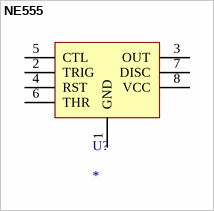
[diagram p0: symbol NE555]
# Altium schematic symbol library MISC89130-9.SchLib: 1 symbol
Pins are listed as number, name and electrical type; pins without a type are passive.


## NE555
designator U?
pins: 1 GND, 2 TRIG, 3 OUT, 4 RST, 5 CTL, 6 THR, 7 DISC, 8 VCC